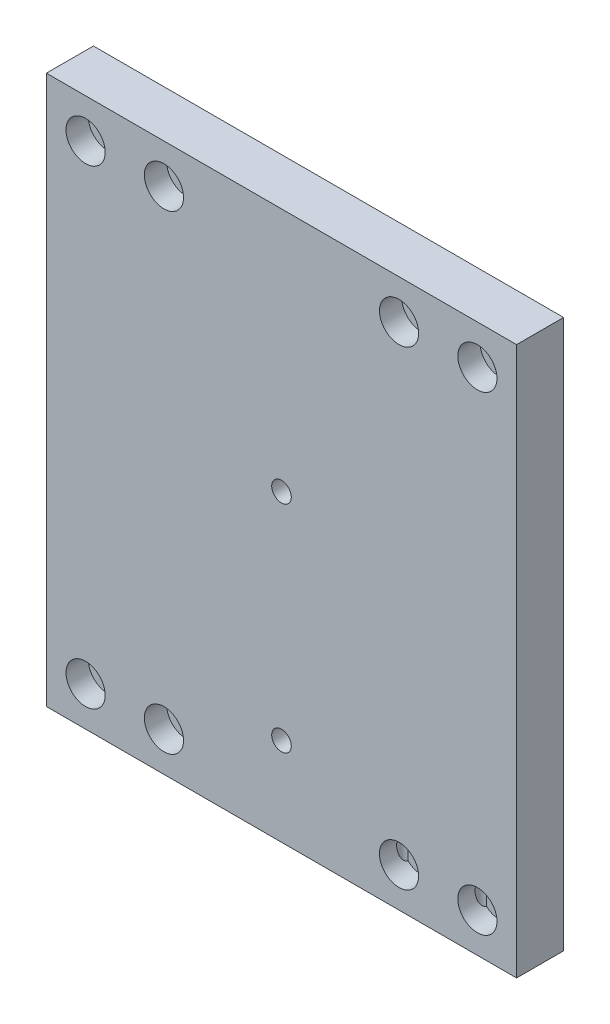
SolidWorks part; units mm, degrees
material "6061 合金"
ref_plane "前视基准面" through (0, 0, 0) normal (0, 0, 1) x (1, 0, 0)
ref_plane "上视基准面" through (0, 0, 0) normal (0, 1, 0) x (1, 0, 0)
ref_plane "右视基准面" through (0, 0, 0) normal (1, 0, 0) x (0, 0, -1)
sketch "草图1" plane through (0, 0, 0) normal (0, 0, 1) x (1, 0, 0)
  line L1 (60, -70) -> (-60, -70)
  line L2 (60, -70) -> (60, 70)
  line L3 (60, 70) -> (-60, 70)
  line L4 (-60, -70) -> (-60, 70)
  line L5 (60, -70) -> (-60, 70) construction
  line L6 (60, 70) -> (-60, -70) construction
  point P0 (0, 0)
  dimension "D1" = 120
  dimension "D2" = 140
extrude "凸台-拉伸1" add sketch "草图1" along normal mid plane 12
hole_wizard "M6 螺纹孔1" positions "3D草图2" profile "草图3" tap size "M6" standard "GB"
sketch3d "3D草图2"
  line L0 (60, -70, 6) -> (60, 70, 6) construction
  line L1 (-60, -70, 6) -> (60, -70, 6) construction
  point P0 (0, -47.5, 6)
  point P2 (0, 7.5, 6)
  dimension "D1" = 60
  dimension "D2" = 60
  dimension "D4" = 55
  dimension "D6" = 22.5
sketch "草图3" plane through (0, -47.5, 6) normal (1, 0, 0) x (0, -1, 0)
  line L0 (0, 0) -> (0, 16.5022)
  line L1 (0, 16.5022) -> (2.5, 15)
  line L2 (2.5, 15) -> (2.5, 0)
  line L5 (2.5, 0) -> (0, 0)
  line L10 (0, 16.5022) -> (-2.5, 15) construction
  line L11 (0, -6.35) -> (0, 107.95) construction
  dimension "螺纹孔钻头直径" = 5
  dimension "螺纹孔钻头深度" = 15
  dimension "导头角度" = 118
cosmetic thread "孔螺蚊线1" parameters "D1"=12, "D2"=6
cosmetic thread "孔螺蚊线2" parameters "D1"=12, "D2"=6
hole_wizard "打孔尺寸(%根据)内六角圆柱头螺钉的类型1" positions "3D草图3" profile "草图4" counterbore size "M5" standard "GB"
sketch3d "3D草图3"
  line L0 (-60, 70, 6) -> (-60, -70, 6) construction
  line L1 (60, -70, 6) -> (60, 70, 6) construction
  line L2 (60, 70, 6) -> (-60, 70, 6) construction
  line L3 (-60, -70, 6) -> (60, -70, 6) construction
  point P0 (-50, 60, 6)
  point P2 (-30, 60, 6)
  point P4 (30, 60, 6)
  point P6 (50, 60, 6)
  point P8 (50, -60, 6)
  point P10 (30, -60, 6)
  point P12 (-30, -60, 6)
  point P14 (-50, -60, 6)
  dimension "D1" = 10
  dimension "D2" = 30
  dimension "D3" = 30
  dimension "D4" = 10
  dimension "D5" = 10
  dimension "D6" = 30
  dimension "D7" = 30
  dimension "D8" = 10
  dimension "D9" = 10
  dimension "D10" = 10
  dimension "D11" = 10
  dimension "D12" = 10
  dimension "D13" = 10
  dimension "D14" = 10
  dimension "D15" = 10
  dimension "D16" = 10
sketch "草图4" plane through (-50, 60, 6) normal (1, 0, 0) x (0, -1, 0)
  line L0 (0, 0) -> (0, 16.6524)
  line L1 (0, 16.6524) -> (2.75, 15)
  line L2 (2.75, 15) -> (2.75, 5.7)
  line L3 (2.75, 5.7) -> (5, 5.7)
  line L4 (5, 5.7) -> (5, 0)
  line L5 (5, 0) -> (0, 0)
  line L10 (0, 16.6524) -> (-2.75, 15) construction
  line L11 (0, -6.35) -> (0, 107.95) construction
  dimension "孔直径" = 5.5
  dimension "孔深度" = 15
  dimension "柱形沉头孔直径" = 10
  dimension "柱形沉头孔深度" = 5.7
  dimension "导头角度" = 118
sketch "草图5" plane through (0, 0, -6) normal (0, 0, -1) x (-1, 0, 0)
  line L0 (60, -70) -> (-60, -70) construction
  line L1 (-60, 70) -> (60, 70) construction
  circle A0 centre (0, 60) radius 2.5
  circle A1 centre (0, -60) radius 2.5
  dimension "D1" = 10
  dimension "D3" = 5
  dimension "D4" = 5
  dimension "D2" = 10
extrude "切除-拉伸1" cut sketch "草图5" against normal blind 6
hole_wizard "M4 螺纹孔2" positions "草图12" profile "草图11" tap size "M4" standard "GB"
sketch "草图12" plane through (0, -70, 0) normal (0, -1, 0) x (-1, 0, 0)
  line L0 (-60, -6) -> (-60, 6) construction
  line L1 (60, 6) -> (-60, 6) construction
  point P0 (-25, 0)
  point P2 (-45, 0)
  dimension "D1" = 20
  dimension "D2" = 15
  dimension "D3" = 6
sketch "草图11" plane through (25, -70, 0) normal (1, 0, 0) x (0, 0, -1)
  line L0 (0, 0) -> (0, 11.0914)
  line L1 (0, 11.0914) -> (1.65, 10.1)
  line L2 (1.65, 10.1) -> (1.65, 0)
  line L5 (1.65, 0) -> (0, 0)
  line L10 (0, 11.0914) -> (-1.65, 10.1) construction
  line L11 (0, -6.35) -> (0, 107.95) construction
  dimension "螺纹孔钻头直径" = 3.3
  dimension "螺纹孔钻头深度" = 10.1
  dimension "导头角度" = 118
cosmetic thread "孔螺蚊线5" parameters "D1"=8, "D2"=4
cosmetic thread "孔螺蚊线6" parameters "D1"=8, "D2"=4
mirror "镜向1" about plane through (0, 0, 0) normal (1, 0, 0) of "M4 螺纹孔2"
